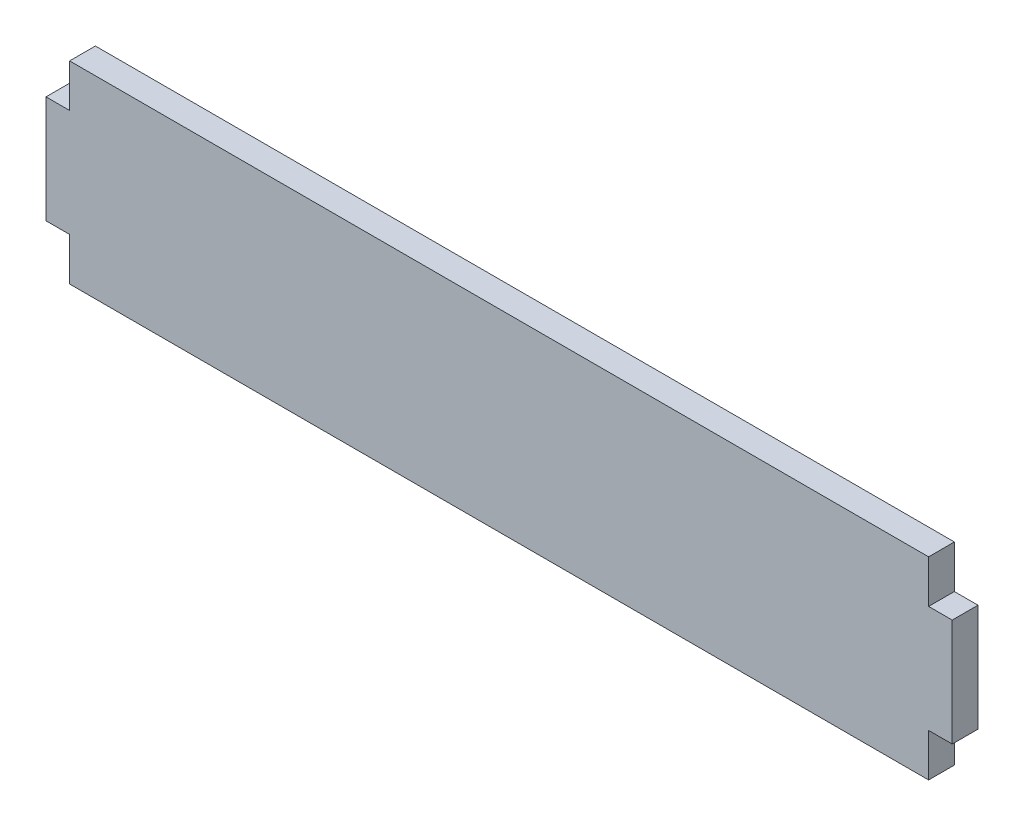
from build123d import *

# Parameters (mm, degrees)
BOSS_EXTRUDE1_DEPTH = 3


with BuildPart() as part:
    # Sketch1 → Boss-Extrude1 (new, symmetric)
    with BuildSketch(Plane.XY):
        Polygon((43.6, -110), (-156.4, -110), (-156.4, -100), (-161.9, -100), (-161.9, -75), (-156.4, -75), (-156.4, -65), (43.6, -65), (43.6, -75), (49.1, -75), (49.1, -100), (43.6, -100), align=None)
    extrude(amount=BOSS_EXTRUDE1_DEPTH, both=True)


solid = part.part
